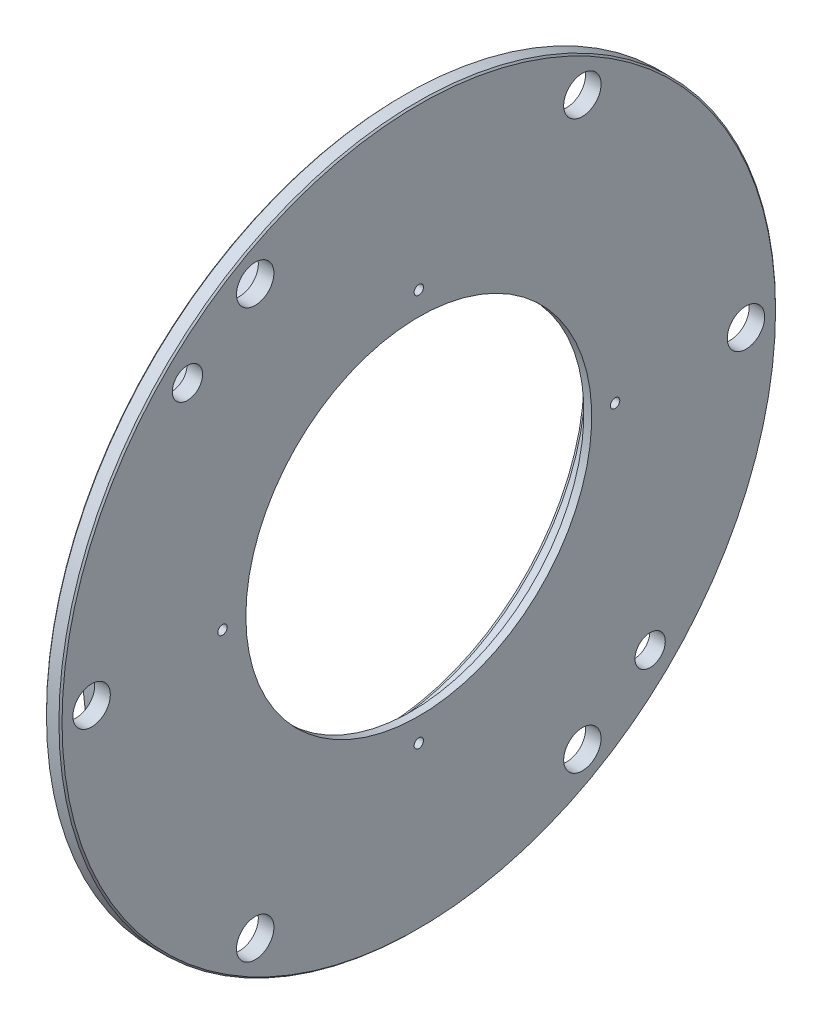
SolidWorks part; units mm, degrees
material "Q235A "
ref_plane "Front Plane" through (0, 0, 0) normal (0, 0, 1) x (1, 0, 0)
ref_plane "Top Plane" through (0, 0, 0) normal (0, 1, 0) x (1, 0, 0)
ref_plane "Right Plane" through (0, 0, 0) normal (1, 0, 0) x (0, 0, -1)
sketch "Sketch1" plane through (0, 0, 0) normal (0, 0, 1) x (1, 0, 0)
  line L0 (0, 111) -> (0, 230)
  line L1 (0, 230) -> (-10, 230)
  line L2 (-10, 230) -> (-10, 190)
  line L3 (-10, 190) -> (-27, 190)
  line L4 (-27, 190) -> (-27, 111)
  line L5 (-27, 111) -> (0, 111)
  line L6 (-73.5631, 0) -> (51.9985, 0) construction
  dimension "D1" = 230
  dimension "D2" = 190
  dimension "D3" = 111
  dimension "D4" = 10
  dimension "D5" = 27
  dimension "D6" = 0
revolve "Revolve1" add sketch "Sketch1" angle 360 about L6
sketch "Sketch3" plane through (0, 0, 0) normal (1, 0, 0) x (0, 0, -1)
  line L0 (-285.3092, 0) -> (277.0751, 0) construction
  line L1 (0, 304.1322) -> (0, -319.5463) construction
  circle A0 centre (0, 0) radius 210 construction
  circle A1 centre (-210, 0) radius 12
  dimension "D1" = 420
  dimension "D2" = 24
extrude "Cut-Extrude1" cut sketch "Sketch3" against normal through all
pattern_circular "CirPattern1" count 6 over 360 about axis through (0, 0, 0) along (1, 0, 0) of "Cut-Extrude1"
sketch "Sketch4" plane through (0, 0, 0) normal (1, 0, 0) x (0, 0, -1)
  line L0 (0, 0) -> (-325.6559, 0) construction
  circle A0 centre (0, 0) radius 126 construction
  circle A1 centre (-126, 0) radius 3
  dimension "D1" = 252
  dimension "D2" = 6
  dimension "D3" = 126
extrude "Cut-Extrude5" cut sketch "Sketch4" against normal through all
pattern_circular "CirPattern2" count 4 over 360 about axis through (0, 0, 0) along (1, 0, 0) of "Cut-Extrude5"
sketch "Sketch5" plane through (-27, 0, 0) normal (-1, 0, 0) x (0, 0, 1)
  circle A0 centre (0, 0) radius 130
  dimension "D1" = 260
extrude "Cut-Extrude6" cut sketch "Sketch5" against normal blind 22
sketch "Sketch6" plane through (-27, 0, 0) normal (-1, 0, 0) x (0, 0, 1)
  circle A0 centre (0, 0) radius 175
  dimension "D1" = 350
extrude "Cut-Extrude7" cut sketch "Sketch6" against normal blind 2
chamfer "Chamfer2" distance 2 angle 30 1 edges at (-25, 0, 130)
chamfer "Chamfer3" distance 1 angle 45 3 edges at (0, 0, 230) (-10, 0, 230) (-27, 0, 190)
hole_wizard "7/8-9 Tapped Hole1" positions "3DSketch3" profile "Sketch10" tap size "7/8-9" standard "Ansi Inch" end condition through all
sketch3d "3DSketch3"
  circle A0 centre (0, 181.8653, 105) radius 12 construction
  point P0 (0, 148.4924, 148.4924)
  point P6 (12, 181.8653, 105)
  dimension "D1" = 210
  dimension "D2" = 54.821
sketch "Sketch10" plane through (0, 148.4924, 148.4924) normal (0, 1, 0) x (0, 0, -1)
  line L0 (0, 0) -> (0, 27)
  line L1 (0, 27) -> (9.7231, 27)
  line L2 (9.7231, 27) -> (9.7231, 0)
  line L5 (9.7231, 0) -> (0, 0)
  line L11 (0, -6.35) -> (0, 107.95) construction
  dimension "通孔螺纹孔钻头直径" = 19.4462
  dimension "通孔螺纹孔钻头深度" = 27
cosmetic thread "CosmeticThread3" parameters "D2"=22.225
pattern_circular "CirPattern4" count 2 over 360 about axis through (0, 0, 0) along (1, 0, 0) of "7/8-9 Tapped Hole1"
